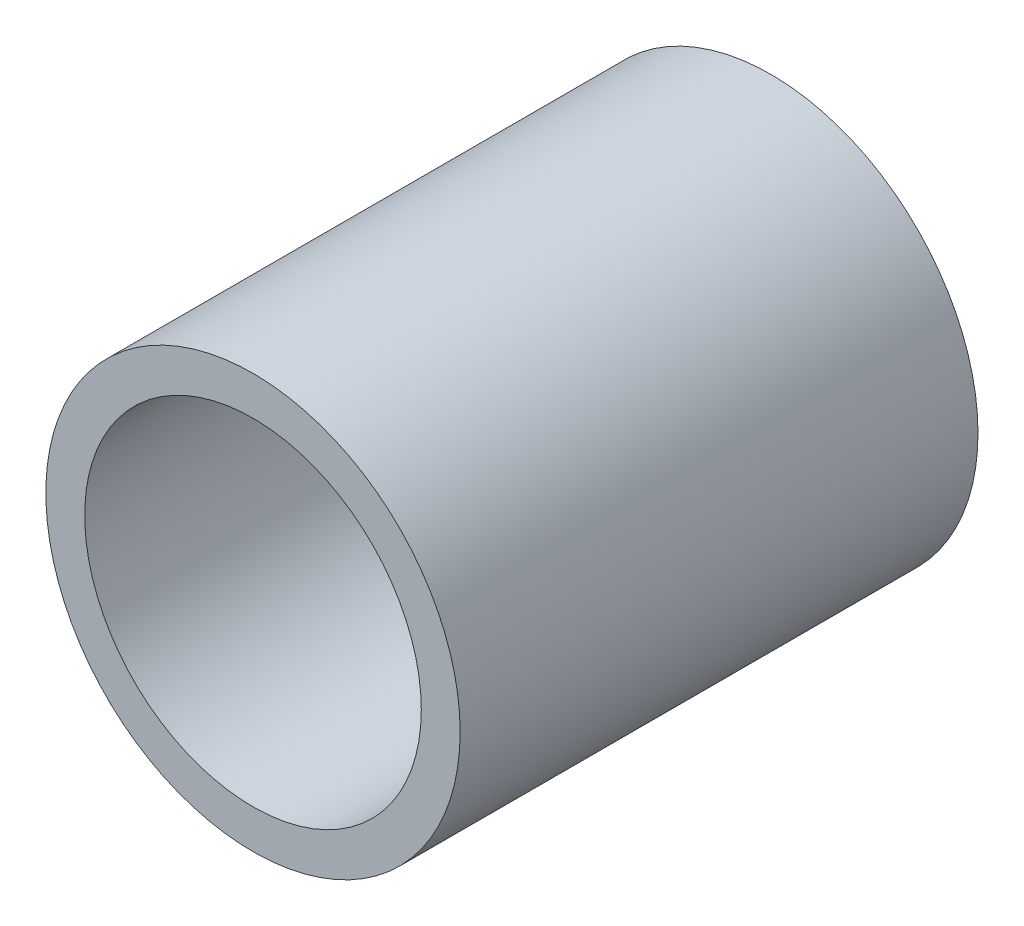
SolidWorks part; units mm, degrees
material "PP 共聚物"
ref_plane "前视基准面" through (0, 0, 0) normal (0, 0, 1) x (1, 0, 0)
ref_plane "上视基准面" through (0, 0, 0) normal (0, 1, 0) x (1, 0, 0)
ref_plane "右视基准面" through (0, 0, 0) normal (1, 0, 0) x (0, 0, -1)
sketch "草图1" plane through (0, 0, 0) normal (0, 0, 1) x (1, 0, 0)
  circle A0 centre (0, 0) radius 16
  dimension "D1" = 32
extrude "拉伸-薄壁1" add sketch "草图1" along normal blind 40 thin thin type one direction reverse wall 3
